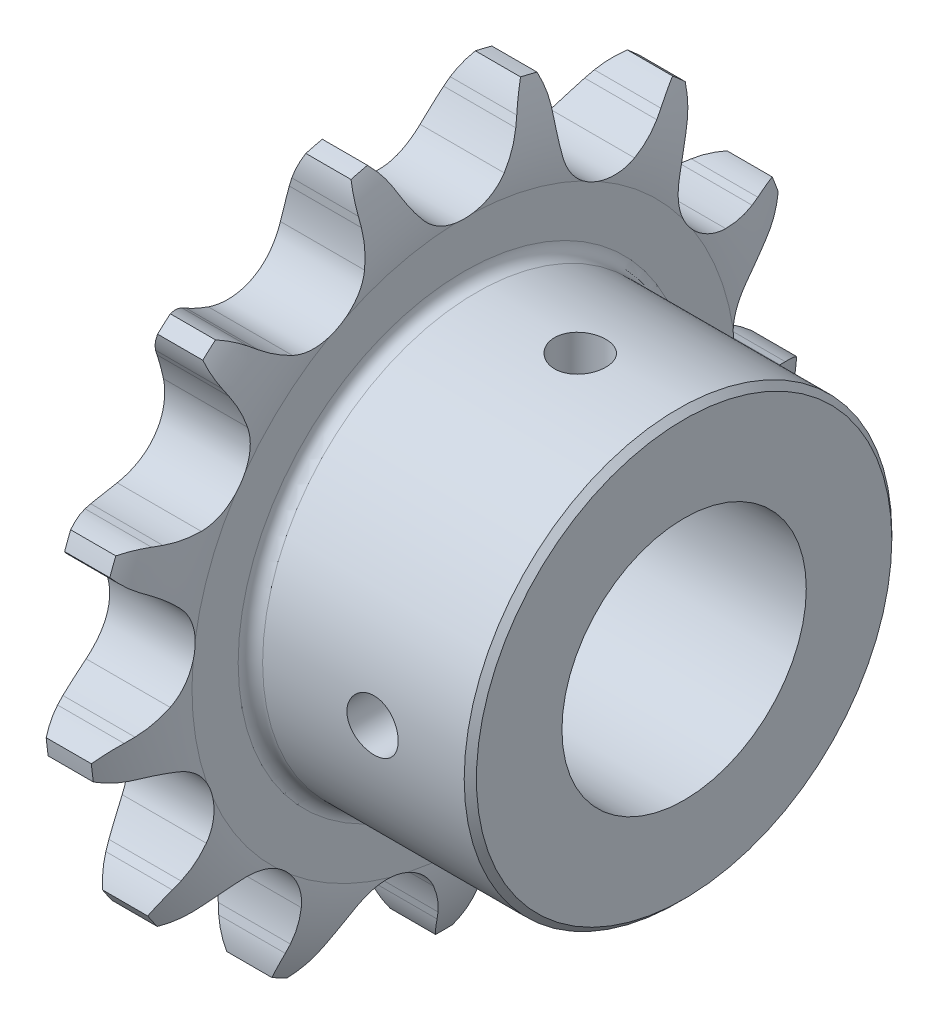
SolidWorks part; units mm, degrees
ref_plane "前视基准面" through (0, 0, 0) normal (0, 0, 1) x (1, 0, 0)
ref_plane "上视基准面" through (0, 0, 0) normal (0, 1, 0) x (1, 0, 0)
ref_plane "右视基准面" through (0, 0, 0) normal (1, 0, 0) x (0, 0, -1)
sketch "草图1" plane through (0, 0, 0) normal (0, 0, 1) x (1, 0, 0)
  line L0 (-6.35, 0) -> (6.35, 0) construction
  line L3 (-3.5, 10) -> (-3.5, 22.279)
  line L4 (-1.849, 29) -> (1.849, 29)
  line L5 (3.5, 22.279) -> (3.5, 10)
  line L8 (3.5, 10) -> (-3.5, 10)
  line L9 (0, 0) -> (0, 29) construction
  line L10 (-2.923, 26.534) -> (2.923, 26.534) construction
  line L11 (-2.923, -26.534) -> (2.923, -26.534) construction
  line L12 (6.35, 0) -> (19.35, 0) construction
  line L13 (-3.5, 22.279) -> (3.7984, 22.279) construction
  line L14 (-3.5, -22.279) -> (3.7984, -22.279) construction
  line L15 (19.35, 0) -> (27.86, 0) construction
  line L16 (27.86, 0) -> (39.67, 0) construction
  line L17 (39.67, 0) -> (47.42, 0) construction
  line L18 (47.42, 0) -> (61.34, 0) construction
  arc A0 (-1.849, 29) -> (-3.5, 22.279) centre (9.1922, 22.7245) ccw
  arc A1 (1.849, 29) -> (3.5, 22.279) centre (-9.1922, 22.7245) cw
  point P30 (3.5, 19)
  point P33 (-3.5, 19)
  dimension "D1" = 3.279
  dimension "rx" = 12.7
  dimension "d" = 53.068
  dimension "p" = 12.7
  dimension "z" = 13
  dimension "da" = 58
  dimension "df" = 44.558
  dimension "dr" = 8.51
  dimension "dk" = 20
  dimension "h" = 11.81
  dimension "bf1" = 7
  dimension "b1" = 7.75
  dimension "ba" = 1.651
  dimension "pt" = 13.92
revolve "旋转1" add sketch "草图1" angle 360 about L0
sketch "草图2" plane through (0, 0, 0) normal (1, 0, 0) x (0, 0, -1)
  line L0 (0, 0) -> (0, 29) construction
  line L1 (0, 0) -> (-6.9402, 28.1573) construction
  line L2 (0, 0) -> (-13.477, 25.6782) construction
  line L3 (3.3327, 23.7754) -> (-2.594, 28.6811) construction
  line L4 (4.7695, 26.0075) -> (-5.2445, 30.875) construction
  line L5 (0, 0) -> (6.9402, 28.1573) construction
  line L6 (4.7695, 26.0075) -> (5.0769, 26.6399)
  line L7 (-4.7695, 26.0075) -> (-5.0769, 26.6399)
  circle A0 centre (0, 0) radius 29 construction
  arc A1 (3.3327, 23.7754) -> (-3.3327, 23.7754) centre (0, 26.534) cw
  arc A2 (3.3327, 23.7754) -> (4.7695, 26.0075) centre (-5.2445, 30.875) ccw
  arc A3 (6.2635, 28.3155) -> (5.0769, 26.6399) centre (10.7415, 23.8864) ccw
  arc A4 (-3.3327, 23.7754) -> (-4.7695, 26.0075) centre (5.2445, 30.875) cw
  arc A5 (-6.2635, 28.3155) -> (-5.0769, 26.6399) centre (-10.7415, 23.8864) cw
  arc A7 (6.2635, 28.3155) -> (-6.2635, 28.3155) centre (0, 0) ccw
  dimension "r1" = 4.3263
  dimension "r3" = 6.2984
  dimension "D1" = 27.692
  dimension "D2" = 13.846
  dimension "α/2" = 50.385
  dimension "M" = 5.2445
  dimension "T" = 4.341
  dimension "β" = 13.692
  dimension "γ/2" = 12.077
  dimension "bc" = 0.7031
extrude "切除-拉伸1" cut sketch "草图2" against normal mid plane 9.2773
pattern_circular "阵列(圆周)1" count 13 over 360 about axis through (0, 0, 0) along (1, 0, 0) of "切除-拉伸1"
sketch "草图3" plane through (3.5, 0, 0) normal (1, 0, 0) x (0, 0, -1)
  circle A0 centre (0, 0) radius 17.5
  circle A1 centre (0, 0) radius 10 construction
  circle A2 centre (0, 0) radius 10
  dimension "D1" = 35
extrude "凸台-拉伸1" add sketch "草图3" along normal blind 18
sketch "草图4" plane through (21.5, 0, 0) normal (1, 0, 0) x (0, 0, -1)
  line L0 (0, 0) -> (0, 27.3022) construction
  line L2 (-3, 7.2) -> (3, 7.2)
  line L3 (-3, 7.2) -> (-3, 12.8)
  line L4 (-3, 12.8) -> (3, 12.8)
  line L5 (3, 7.2) -> (3, 12.8)
  line L6 (-3, 7.2) -> (3, 12.8) construction
  line L7 (-3, 12.8) -> (3, 7.2) construction
  circle A0 centre (0, 0) radius 10 construction
  point P3 (0, 10)
  dimension "D1" = 6
  dimension "D2" = 5.6
fillet "圆角1" radius 1 1 edges at (3.5, 0, 17.5)
chamfer "倒角1" distance 0.5 angle 45 1 edges at (21.5, 0, -17.5)
ref_plane "基准面1" through (0, 17.5, 0) normal (0, 1, 0) x (1, 0, 0)
hole_wizard "M5 螺纹孔1" positions "草图6" profile "草图5" tap size "M5" standard "Iso"
sketch "草图6" plane through (0, 17.5, 0) normal (0, 1, 0) x (1, 0, 0)
  line L0 (21.5, 0) -> (13, 0) construction
  line L1 (21.5, -17) -> (21.5, 17) construction
  point P2 (13, 0)
  dimension "D1" = 8.5
sketch "草图5" plane through (13, 17.5, 0) normal (1, 0, 0) x (0, 0, 1)
  line L0 (0, 0) -> (0, 13.6618)
  line L1 (0, 13.6618) -> (2.1, 12.4)
  line L2 (2.1, 12.4) -> (2.1, 0)
  line L5 (2.1, 0) -> (0, 0)
  line L10 (0, 13.6618) -> (-2.1, 12.4) construction
  line L11 (0, -6.35) -> (0, 107.95) construction
  dimension "螺纹孔钻头直径" = 4.2
  dimension "螺纹孔钻头深度" = 12.4
  dimension "导头角度" = 118
cosmetic thread "孔螺蚊线1" parameters "D1"=4.7, "D2"=5
ref_plane "基准面2" through (0, 0, 17.5) normal (0, 0, 1) x (1, 0, 0)
hole_wizard "M5 螺纹孔2" positions "草图8" profile "草图7" tap size "M5" standard "Iso"
sketch "草图8" plane through (0, 0, 17.5) normal (0, 0, 1) x (1, 0, 0)
  line L0 (21.5, 0) -> (13.5, 0)
  line L1 (21.5, -17) -> (21.5, 17) construction
  point P1 (13.5, 0)
  dimension "D1" = 8
sketch "草图7" plane through (13.5, 0, 17.5) normal (1, 0, 0) x (0, -1, 0)
  line L0 (0, 0) -> (0, 13.6618)
  line L1 (0, 13.6618) -> (2.1, 12.4)
  line L2 (2.1, 12.4) -> (2.1, 0)
  line L5 (2.1, 0) -> (0, 0)
  line L10 (0, 13.6618) -> (-2.1, 12.4) construction
  line L11 (0, -6.35) -> (0, 107.95) construction
  dimension "螺纹孔钻头直径" = 4.2
  dimension "螺纹孔钻头深度" = 12.4
  dimension "导头角度" = 118
cosmetic thread "孔螺蚊线2" parameters "D1"=7.723, "D2"=5
sketch "草图9" plane through (-3.5, 0, 0) normal (-1, 0, 0) x (0, 0, 1)
  circle A0 centre (0, 0) radius 26.54
  dimension "D1" = 53.08
